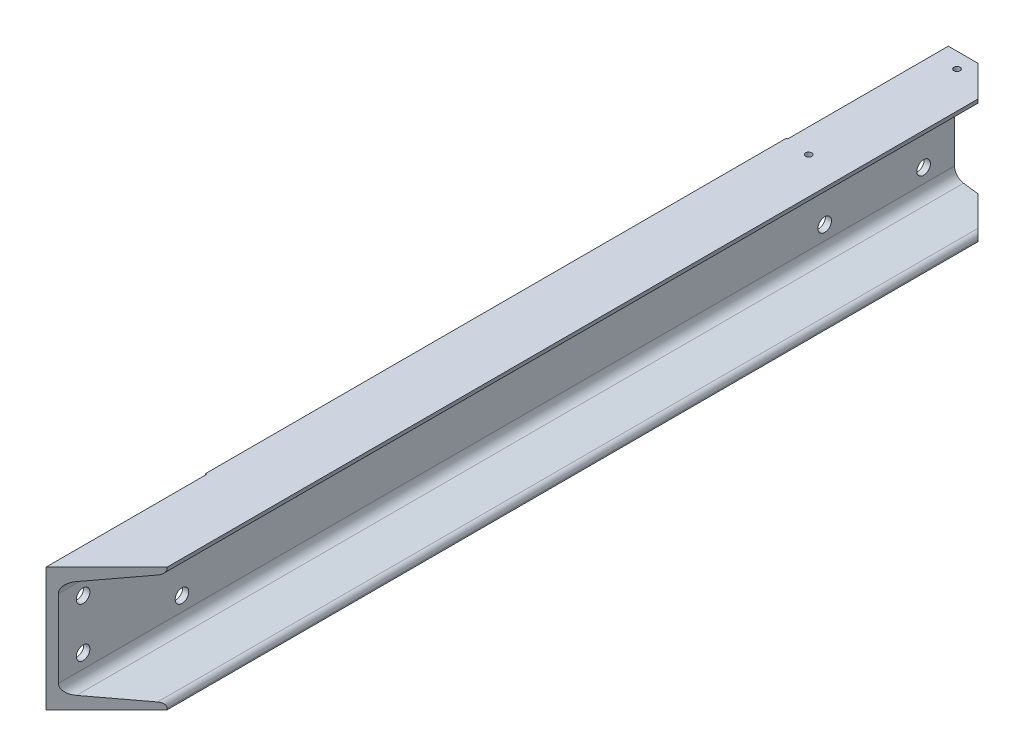
from build123d import *

# Parameters (mm, degrees)
BOSS_EXTRUDE1_DEPTH   = 750
CUT_EXTRUDE1_DEPTH    = 730
SKETCH3_W             = 246.792493201
SKETCH3_H             = 411.477698095
CUT_EXTRUDE2_DEPTH    = 1
SKETCH4_R             = 5.5
CUT_EXTRUDE3_DEPTH    = 10
M6_TAPPED_HOLE3_D     = 5
M6_TAPPED_HOLE3_DEPTH = 15
M6_TAPPED_HOLE3_TIP   = 1.502151548


with BuildPart() as part:
    # Sketch1 → Boss-Extrude1 (new body)
    with BuildSketch(Plane.XY):
        with BuildLine():
            Line((0, 0), (0, -100))
            Line((0, -100), (50, -100))
            Line((50, -100), (50, -98.925311188))
            ThreePointArc((50, -98.925311188), (48.896193111, -95.973045557), (46.126278954, -94.469104878))
            Line((46.126278954, -94.469104878), (13.317028642, -89.858065454))
            ThreePointArc((13.317028642, -89.858065454), (8.084968568, -87.017288616), (6, -81.440786869))
            Line((6, -81.440786869), (6, -18.559213131))
            ThreePointArc((6, -18.559213131), (8.084968568, -12.982711384), (13.317028642, -10.141934546))
            Line((13.317028642, -10.141934546), (46.126278954, -5.530895122))
            ThreePointArc((46.126278954, -5.530895122), (48.896193111, -4.026954443), (50, -1.074688812))
            Line((50, -1.074688812), (50, 0))
            Line((50, 0), (0, 0))
        make_face()
    extrude(amount=BOSS_EXTRUDE1_DEPTH)

    # Sketch2 → Cut-Extrude1 (cut)
    with BuildSketch(Plane(origin=(0, 0, 0), x_dir=(1, 0, 0), z_dir=(0, 1, 0))):
        Polygon((258.992644717, -472.007355283), (0, -731), (-59.777153602, -772.262203455), (30.841373369, -818.159898935), (45.044802943, -785.872759949), (459.456990019, -587.675626999), align=None)
        Polygon((25, 0), (50, -25), (50, 48.41721094), align=None)
    extrude(amount=-CUT_EXTRUDE1_DEPTH, mode=Mode.SUBTRACT)

    # Sketch3 → Cut-Extrude2 (cut)
    with BuildSketch(Plane.ZY):
        Polygon((130, 38.70177923), (130, -162.725177772), (-125.633599865, -119.606257313), (-100.418312462, 29.884375145), align=None)
        with Locations((723.396246601, 67.037069817)):
            Rectangle(SKETCH3_W, SKETCH3_H)
    extrude(amount=-CUT_EXTRUDE2_DEPTH, mode=Mode.SUBTRACT)

    # Sketch4 → Cut-Extrude3 (cut)
    with BuildSketch(Plane.ZY.offset(-1)):
        with Locations(Location((25, -30, 0), (0, 0, 270))):
            Circle(SKETCH4_R)
        with Locations(Location((105, -30, 0), (0, 0, 270))):
            Circle(SKETCH4_R)
        with Locations(Location((25, -70, 0), (0, 0, 270))):
            Circle(SKETCH4_R)
        with Locations(Location((105, -70, 0), (0, 0, 270))):
            Circle(SKETCH4_R)
        with Locations(Location((625, -30, 0), (0, 0, 270))):
            Circle(SKETCH4_R)
        with Locations(Location((705, -70, 0), (0, 0, 270))):
            Circle(SKETCH4_R)
        with Locations(Location((625, -70, 0), (0, 0, 270))):
            Circle(SKETCH4_R)
        with Locations(Location((705, -30, 0), (0, 0, 270))):
            Circle(SKETCH4_R)
    extrude(amount=-CUT_EXTRUDE3_DEPTH, mode=Mode.SUBTRACT)

    # M6 Tapped Hole3
    with Locations(Plane(origin=(0, 0, 0), x_dir=(1, 0, 0), z_dir=(0, 1, 0))):
        with Locations((20.5, -12.5), (20.5, -132.5)):
            Hole(M6_TAPPED_HOLE3_D / 2, depth=M6_TAPPED_HOLE3_DEPTH)
            with Locations((0, 0, -(M6_TAPPED_HOLE3_DEPTH + M6_TAPPED_HOLE3_TIP / 2))):  # 118° drill point
                Cone(0, M6_TAPPED_HOLE3_D / 2, M6_TAPPED_HOLE3_TIP, mode=Mode.SUBTRACT)


solid = part.part
